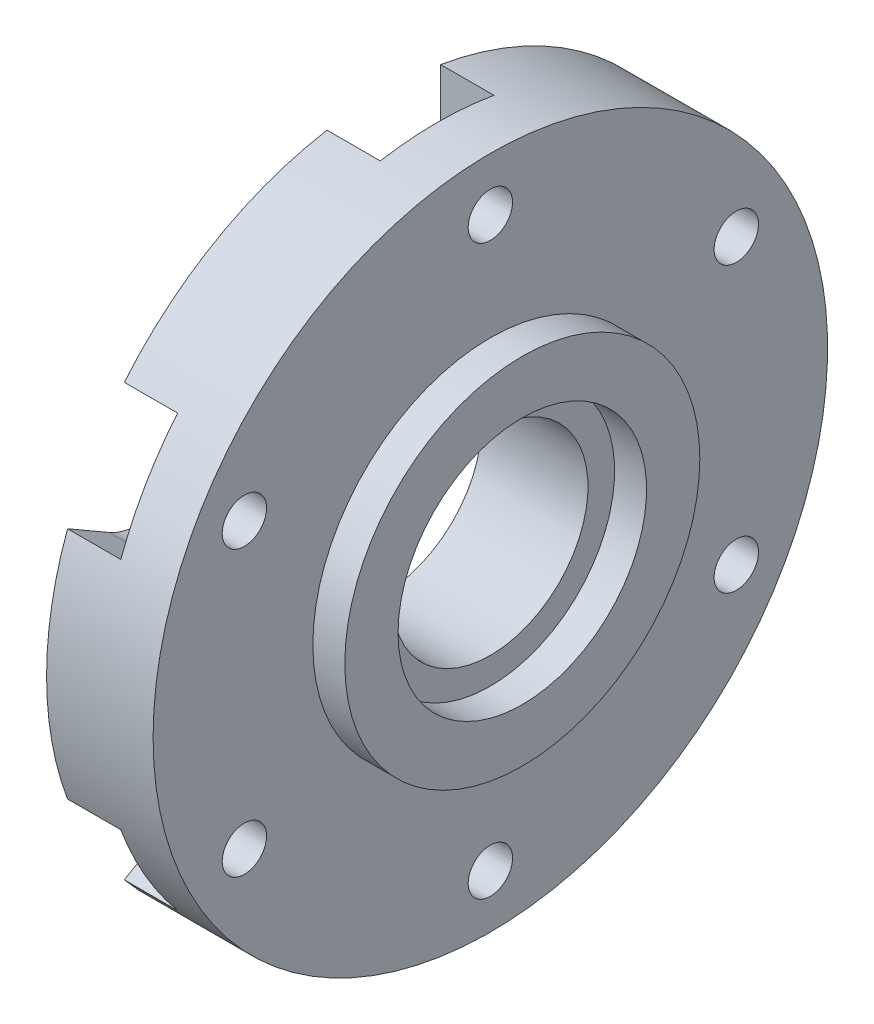
from build123d import *

# Parameters (mm, degrees)
SKETCH_2_R               = 6.25
CUT_EXTRUDE_1_DEPTH      = 140.896390232
PATTERN_CIRCULAR_1_COUNT = 6
SKETCH_3_R               = 27.5
CUT_EXTRUDE_2_DEPTH      = 140.896390232
CUT_EXTRUDE_START        = -15
CUT_EXTRUDE_3_DEPTH      = 15
PATTERN_CIRCULAR_2_COUNT = 6
PATTERN_CIRCULAR_3_COUNT = 6


with BuildPart() as part:
    # 草图1 → 旋转1 (revolve)
    with BuildSketch(Plane.XY, mode=Mode.PRIVATE) as revolve_1_sk:
        Polygon((0, 0), (0, 95), (30, 95), (30, 50), (39, 50), (39, 35), (30, 35), (30, 0), align=None)
    revolve(revolve_1_sk.sketch.rotate(Axis((0, 0, 0), (1, 0, 0)), 90), axis=Axis((0, 0, 0), (1, 0, 0)))

    # 草图2 → 切除-拉伸1 (cut, through all)
    with BuildSketch(Plane.ZY):
        with Locations((0, 80)):
            Circle(SKETCH_2_R)
    cut_extrude_1 = extrude(amount=-CUT_EXTRUDE_1_DEPTH, mode=Mode.SUBTRACT)

    # 阵列(圆周)1: 切除-拉伸1 ×6 about axis
    pattern_circular_1_axis = Axis((0, 0, 0), (1, 0, 0))
    for i in range(1, PATTERN_CIRCULAR_1_COUNT):
        add(cut_extrude_1.rotate(pattern_circular_1_axis, i * 360 / PATTERN_CIRCULAR_1_COUNT), mode=Mode.SUBTRACT)

    # 草图3 → 切除-拉伸2 (cut, through all)
    with BuildSketch(Plane.ZY):
        Circle(SKETCH_3_R)
    extrude(amount=-CUT_EXTRUDE_2_DEPTH, mode=Mode.SUBTRACT)

    # 草图6 → 切除-拉伸3 (cut)
    with BuildSketch(Plane.ZY.offset(CUT_EXTRUDE_START)):
        with BuildLine():
            Line((-16, 80), (-16, 93.642938869))
            ThreePointArc((-16, 93.642938869), (0, 95), (16, 93.642938869))
            Line((16, 93.642938869), (16, 80))
            ThreePointArc((16, 80), (0, 64), (-16, 80))
        make_face()
    cut_extrude_3 = extrude(amount=CUT_EXTRUDE_3_DEPTH, mode=Mode.SUBTRACT)

    # 阵列(圆周)2: 切除-拉伸3 ×6 about axis
    pattern_circular_2_axis = Axis((0, 0, 0), (1, 0, 0))
    for i in range(1, PATTERN_CIRCULAR_2_COUNT):
        add(cut_extrude_3.rotate(pattern_circular_2_axis, i * 360 / PATTERN_CIRCULAR_2_COUNT), mode=Mode.SUBTRACT)

    # 草图8 → M12 螺纹孔1 (revolve, cut)
    with BuildSketch(Plane(origin=(0, 69.282032303, 40), x_dir=(0, 0, 1), z_dir=(0, 1, 0))):
        Polygon((0, 0), (0, 21.064389157), (5.1, 18), (5.1, 0), align=None)
    hole_wizard_m12_1 = revolve(axis=Axis((-6.35, 69.282032303, 40), (1, 0, 0)), mode=Mode.SUBTRACT)

    # 阵列(圆周)3: M12 螺纹孔1 ×6 about axis
    pattern_circular_3_axis = Axis((0, 0, 0), (1, 0, 0))
    for i in range(1, PATTERN_CIRCULAR_3_COUNT):
        add(hole_wizard_m12_1.rotate(pattern_circular_3_axis, i * 360 / PATTERN_CIRCULAR_3_COUNT), mode=Mode.SUBTRACT)


solid = part.part
